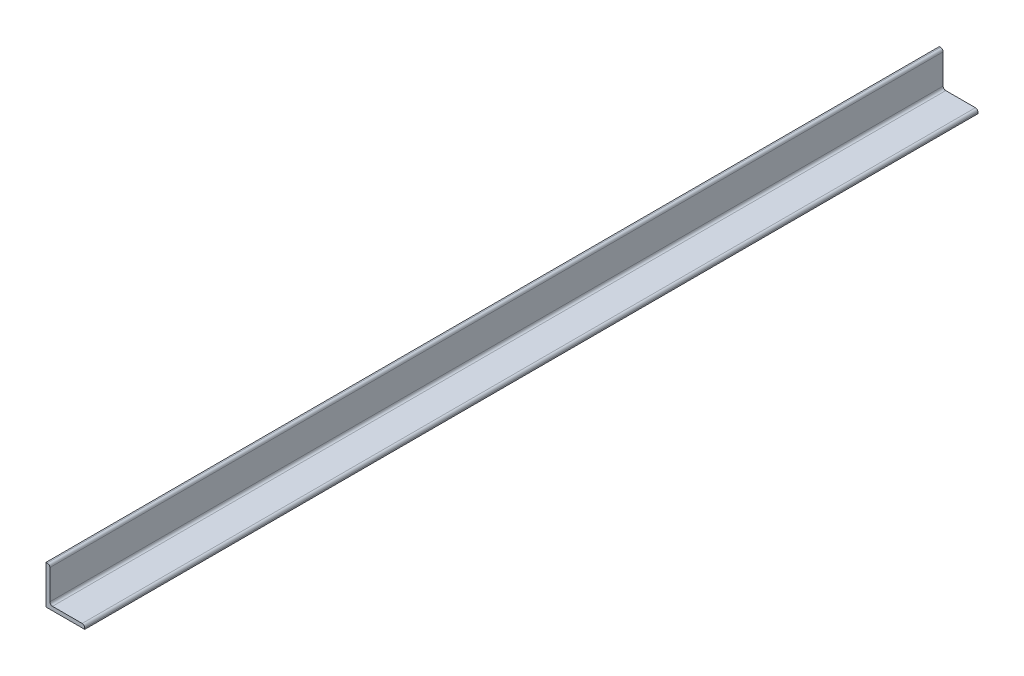
from build123d import *

# Parameters (mm, degrees)
BOSS_EXTRUDE1_DEPTH = 692


with BuildPart() as part:
    # Sketch1 → Boss-Extrude1 (new body)
    with BuildSketch(Plane.XY):
        with BuildLine():
            Line((0, 0), (30, 0))
            Line((30, 0), (30, 1))
            ThreePointArc((30, 1), (29.414213562, 2.414213562), (28, 3))
            Line((28, 3), (5, 3))
            ThreePointArc((5, 3), (3.585786438, 3.585786438), (3, 5))
            Line((3, 5), (3, 28))
            ThreePointArc((3, 28), (2.414213562, 29.414213562), (1, 30))
            Line((1, 30), (0, 30))
            Line((0, 30), (0, 0))
        make_face()
    extrude(amount=BOSS_EXTRUDE1_DEPTH)


solid = part.part
